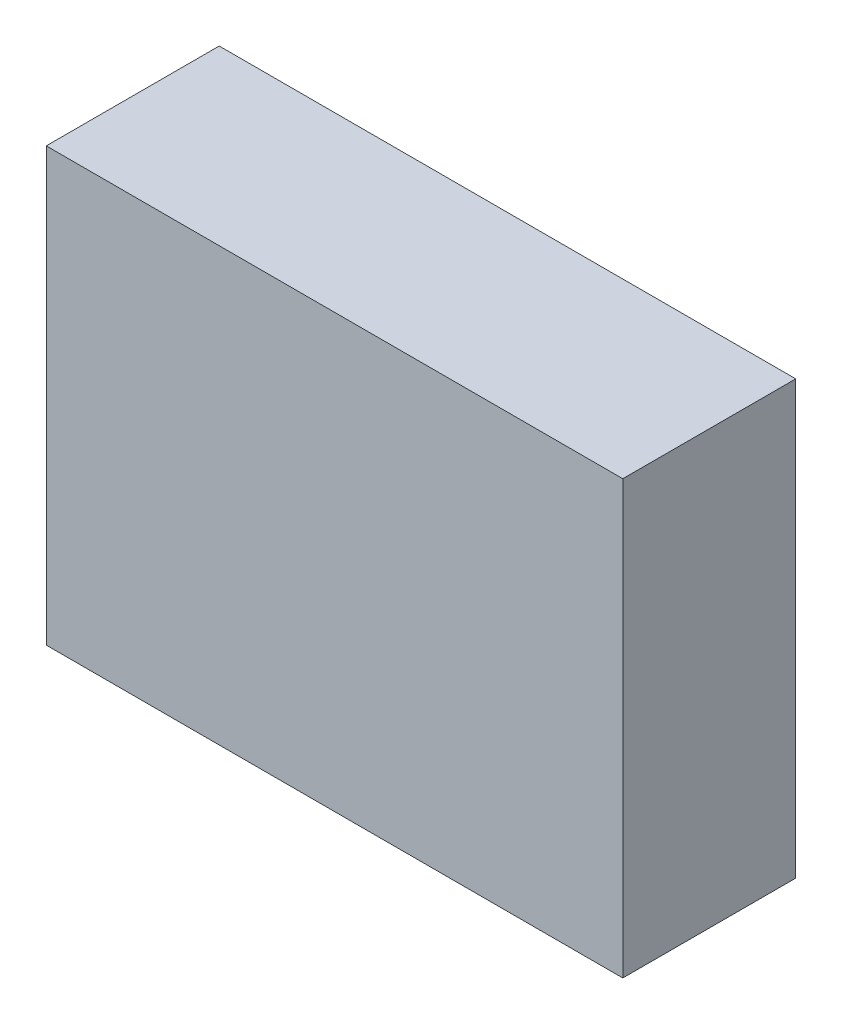
from build123d import *

# Parameters (mm, degrees)
SKETCH_1_W      = 40
SKETCH_1_H      = 30
EXTRUDE_1_DEPTH = 6


with BuildPart() as part:
    # 草图1 → 凸台-拉伸1 (new, symmetric)
    with BuildSketch(Plane.XY):
        Rectangle(SKETCH_1_W, SKETCH_1_H)
    extrude(amount=EXTRUDE_1_DEPTH, both=True)


solid = part.part
